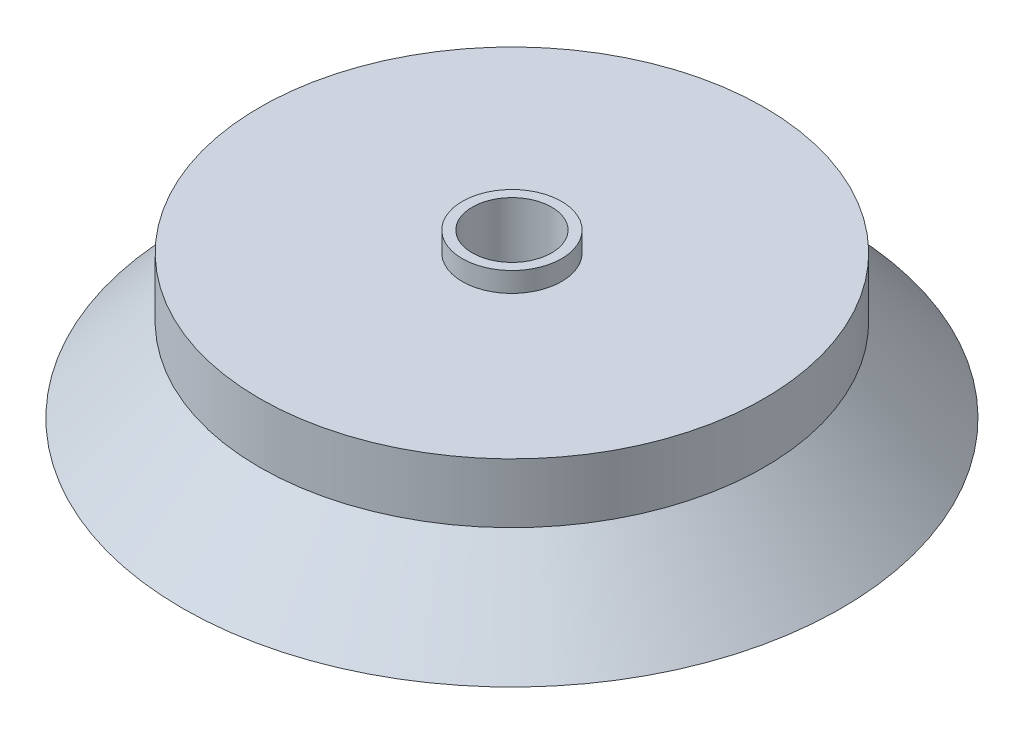
SolidWorks part; units mm, degrees
ref_plane "前视基准面" through (0, 0, 0) normal (0, 0, 1) x (1, 0, 0)
ref_plane "上视基准面" through (0, 0, 0) normal (0, 1, 0) x (1, 0, 0)
ref_plane "右视基准面" through (0, 0, 0) normal (1, 0, 0) x (0, 0, -1)
sketch "草图1" plane through (0, 0, 0) normal (0, 0, 1) x (1, 0, 0)
  line L0 (0, 20.5592) -> (0, -16.1732) construction
  line L1 (-6.25, 17.8136) -> (-5, 17.8136)
  line L2 (-6.25, 17.8136) -> (-6.25, 15.3136)
  line L3 (-6.25, 15.3136) -> (-31.7659, 15.3136)
  line L4 (-31.7659, 15.3136) -> (-31.7659, 7.8136)
  line L5 (-31.7659, 7.8136) -> (-41.5, -2.6864)
  line L6 (-41.5, -2.6864) -> (-38.5, -2.6864)
  line L7 (-38.5, -2.6864) -> (-31.9815, 4.345)
  line L8 (-31.9815, 4.345) -> (-5, 4.345)
  line L9 (-5, 17.8136) -> (-5, 4.345)
  dimension "D1" = 12.5
  dimension "D2" = 1.25
  dimension "D3" = 2.5
  dimension "D4" = 20.5
  dimension "D5" = 10
  dimension "D6" = 77
  dimension "D7" = 3
revolve "旋转1" add sketch "草图1" angle 360 about L0
